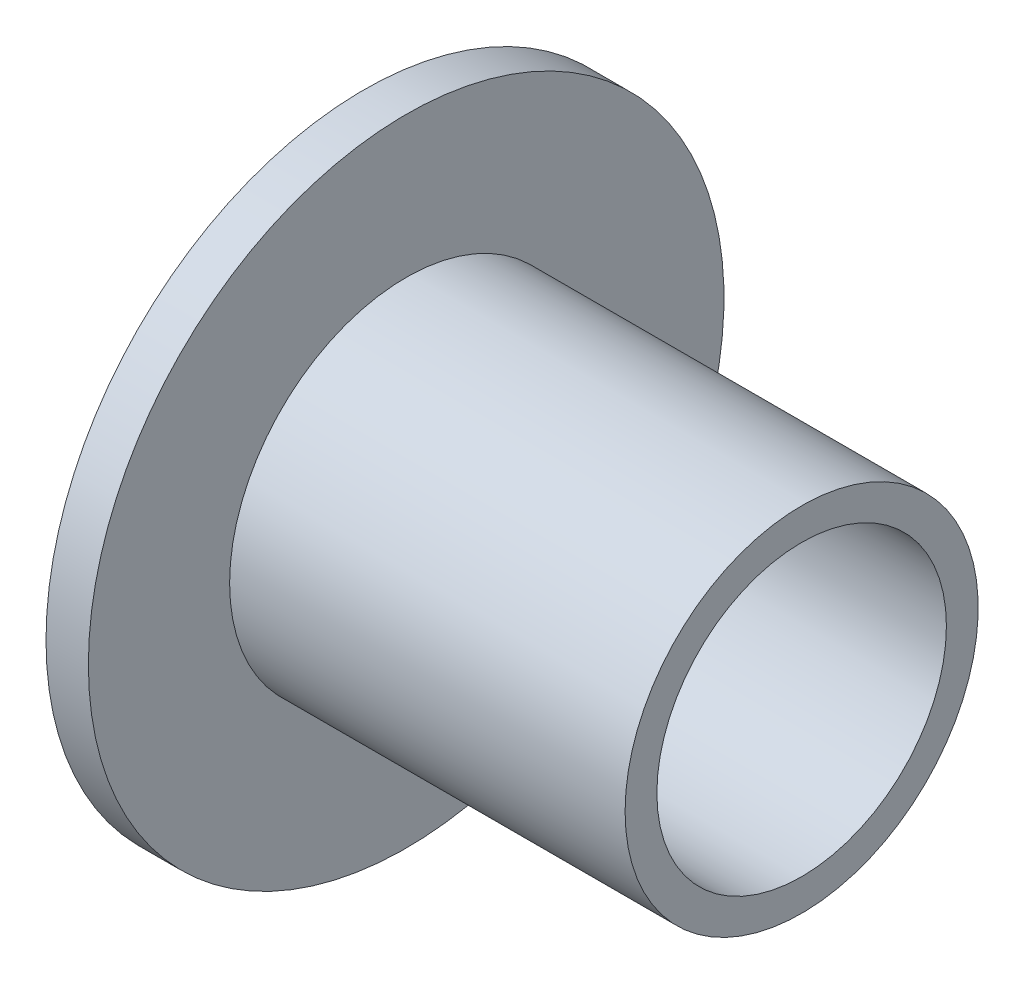
from build123d import *


with BuildPart() as part:
    # 草图1 → 旋转1 (revolve)
    with BuildSketch(Plane.XY, mode=Mode.PRIVATE) as revolve_1_sk:
        Polygon((0, 4.1), (0, 9), (1.2, 9), (1.2, 5), (12.4, 5), (12.4, 4.1), align=None)
    revolve(revolve_1_sk.sketch.rotate(Axis((0, 0, 0), (1, 0, 0)), 90), axis=Axis((0, 0, 0), (1, 0, 0)))


solid = part.part
